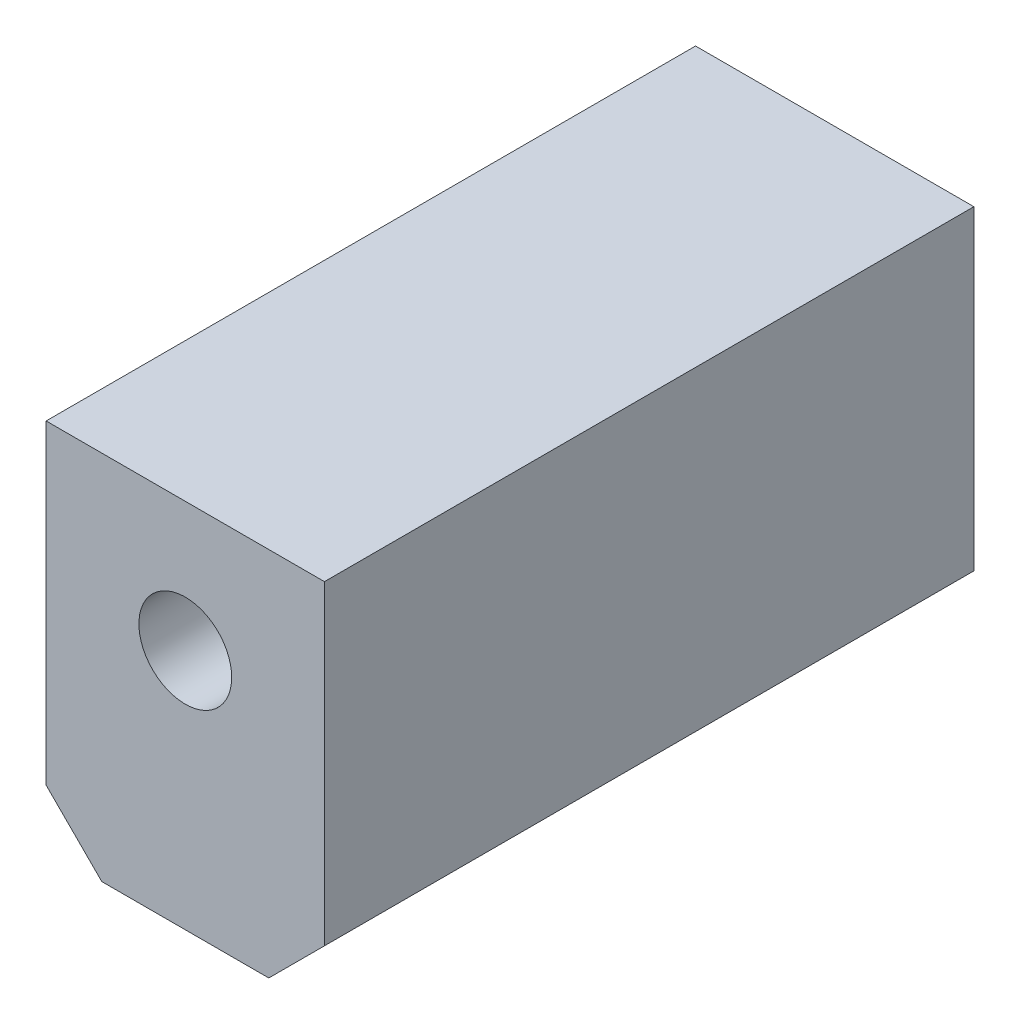
SolidWorks part; units mm, degrees
ref_plane "Front Plane" through (0, 0, 0) normal (0, 0, 1) x (1, 0, 0)
ref_plane "Top Plane" through (0, 0, 0) normal (0, 1, 0) x (1, 0, 0)
ref_plane "Right Plane" through (0, 0, 0) normal (1, 0, 0) x (0, 0, -1)
sketch "Sketch1" plane through (0, 0, 0) normal (0, 0, 1) x (1, 0, 0)
  line L1 (-7.5, 10) -> (7.5, 10)
  line L2 (-7.5, 10) -> (-7.5, -10)
  line L3 (-7.5, -10) -> (7.5, -10)
  line L4 (7.5, 10) -> (7.5, -10)
  line L5 (-7.5, 10) -> (7.5, -10) construction
  line L6 (-7.5, -10) -> (7.5, 10) construction
  point P0 (0, 0)
  dimension "D1" = 15
  dimension "D2" = 20
extrude "Boss-Extrude1" add sketch "Sketch1" along normal mid plane 35
chamfer "Chamfer1" distance 3 angle 45 2 edges at (7.5, -10, 0) (-7.5, -10, 0)
sketch "Sketch2" plane through (0, 0, 17.5) normal (0, 0, 1) x (1, 0, 0)
  line L2 (-4.5, -10) -> (4.5, -10) construction
  point P0 (0, 3.03)
  dimension "D1" = 13.03
hole_wizard "M6 Tapped Hole1" positions "Sketch3" profile "Sketch4" tap size "M6" standard "GB"
sketch "Sketch3" plane through (0, 0, 17.5) normal (0, 0, 1) x (1, 0, 0)
  point P0 (0, 3.03)
sketch "Sketch4" plane through (0, 3.03, 17.5) normal (1, 0, 0) x (0, -1, 0)
  line L0 (0, 0) -> (0, 16.5022)
  line L1 (0, 16.5022) -> (2.5, 15)
  line L2 (2.5, 15) -> (2.5, 0)
  line L5 (2.5, 0) -> (0, 0)
  line L10 (0, 16.5022) -> (-2.5, 15) construction
  line L11 (0, -6.35) -> (0, 107.95) construction
  dimension "螺纹孔钻头直径" = 5
  dimension "螺纹孔钻头深度" = 15
  dimension "导头角度" = 118
cosmetic thread "Cosmetic thread 1"
